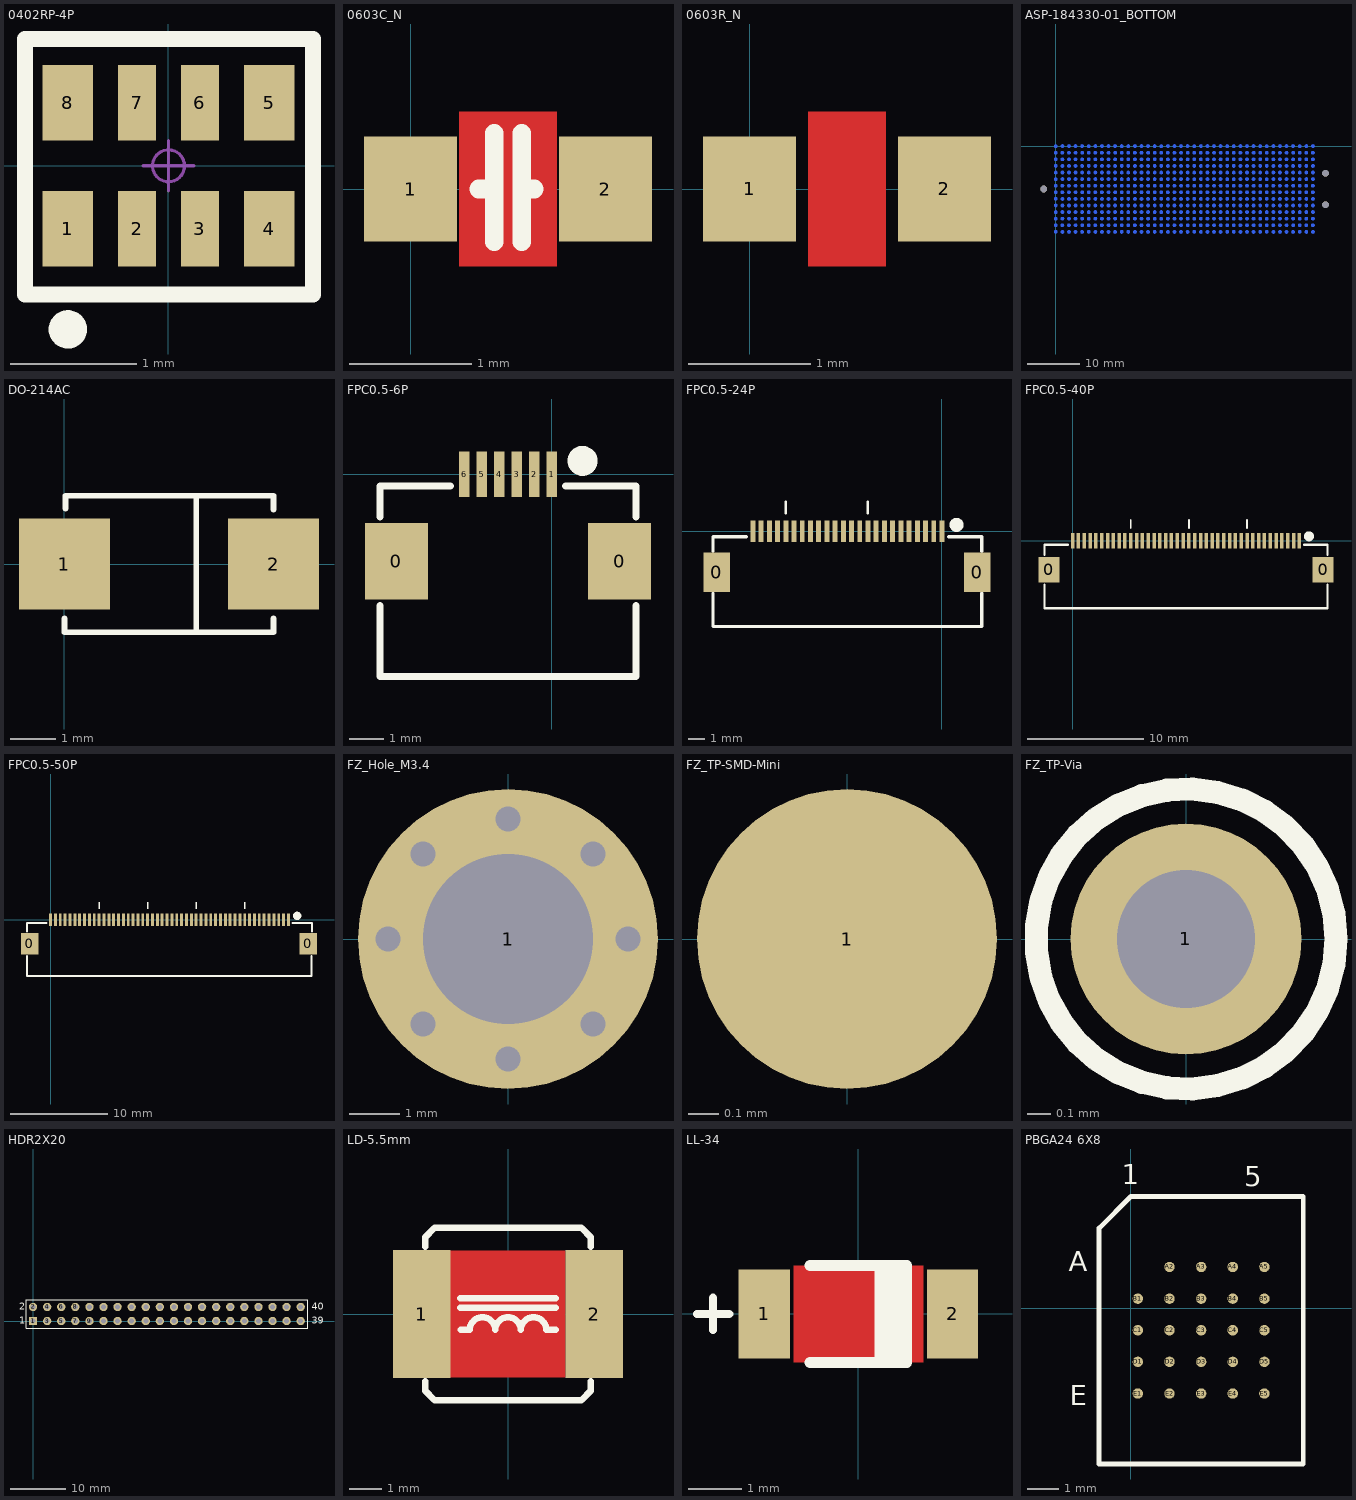
[diagram p0: the footprints below, top view; thin cyan lines are the x and y axes]
# Altium footprint library MISC105414-6.PcbLib: 28 footprints (part 1 of 2)
Each footprint in its own frame and in the unit in brackets; x right, y up, seen from the top. Pads: shape width x height; smd on the part's side, far side on the other; paste and mask are expansions set on the pad; w line width, h text height; cw(c..) or ccw(c..) is an arc to the next point about the centre after c.

## 0402RP-4P [mm] "2mm*1mm*0.45mm(长*宽*厚)"
pads (8):
  rect 0.4x0.6 smd: 1(-0.8,-0.5) 4(0.8,-0.5) 5(0.8,0.5) 8(-0.8,0.5)
  rect 0.3x0.6 smd: 2(-0.25,-0.5) 3(0.25,-0.5) 6(0.25,0.5) 7(-0.25,0.5)
Top Overlay:
  circle w0.152: c-0.8,-1.3 r0.076
  lines w0.127: -1.139,-1.024 -1.139,1.008 1.147,1.008 1.147,-1.024 -1.139,-1.024
Mechanical 15:
  circle w0.025: c0,0 r0.127
  lines w0.025: -0.2,0 0.2,0 ; 0,-0.2 0,0.2
3D body "RCA-8P4R-0402.STEP": height 0.45, standoff 0, extent -1,-0.5 1,0.5

## 0603C_N [mil]
pads (2):
  rect 30x34 smd: 1(-0.01,-0.01) 2(62.99,-0.01)
Top Layer:
  pour cut-out: 15.74,25 47.24,25 47.24,-25 15.74,-25
Top Overlay:
  lines w6: 22,0 27,0 ; 27,-17 27,18 ; 36,-17 36,18 ; 36,0 40,0
3D body "User Library-0603 SMD Capacitor.step": height 12.49, standoff 0.6, extent 0,-15.75 63,15.75

## 0603R_N [mil]
pads (2):
  rect 30x34 smd: 1(0,0) 2(62.99,0)
Top Layer:
  pour cut-out: 19,-25 19,25 44,25 44,-25
3D body "User Library-RESC1608X05N.step": height 17.76, standoff 0, extent 0.01,-16.73 61.03,16.74

## ASP-184330-01_BOTTOM [mm]
pads (560):
  round 0.64 smd far side: A1(0,-2.54) A2(1.27,-2.54) A3(2.54,-2.54) A4(3.81,-2.54) A5(5.08,-2.54) A6(6.35,-2.54) A7(7.62,-2.54) A8(8.89,-2.54) A9(10.16,-2.54) A10(11.43,-2.54) A11(12.7,-2.54) A12(13.97,-2.54) A13(15.24,-2.54) A14(16.51,-2.54) A15(17.78,-2.54) A16(19.05,-2.54) A17(20.32,-2.54) A18(21.59,-2.54) A19(22.86,-2.54) A20(24.13,-2.54) A21(25.4,-2.54) A22(26.67,-2.54) A23(27.94,-2.54) A24(29.21,-2.54) A25(30.48,-2.54) A26(31.75,-2.54) A27(33.02,-2.54) A28(34.29,-2.54) A29(35.56,-2.54) A30(36.83,-2.54) A31(38.1,-2.54) A32(39.37,-2.54) A33(40.64,-2.54) A34(41.91,-2.54) A35(43.18,-2.54) A36(44.45,-2.54) A37(45.72,-2.54) A38(46.99,-2.54) A39(48.26,-2.54) A40(49.53,-2.54) B1(0,-3.81) B2(1.27,-3.81) B3(2.54,-3.81) B4(3.81,-3.81) B5(5.08,-3.81) B6(6.35,-3.81) B7(7.62,-3.81) B8(8.89,-3.81) B9(10.16,-3.81) B10(11.43,-3.81) B11(12.7,-3.81) B12(13.97,-3.81) B13(15.24,-3.81) B14(16.51,-3.81) B15(17.78,-3.81) B16(19.05,-3.81) B17(20.32,-3.81) B18(21.59,-3.81) B19(22.86,-3.81) B20(24.13,-3.81) B21(25.4,-3.81) B22(26.67,-3.81) B23(27.94,-3.81) B24(29.21,-3.81) B25(30.48,-3.81) B26(31.75,-3.81) B27(33.02,-3.81) B28(34.29,-3.81) B29(35.56,-3.81) B30(36.83,-3.81) B31(38.1,-3.81) B32(39.37,-3.81) B33(40.64,-3.81) B34(41.91,-3.81) B35(43.18,-3.81) B36(44.45,-3.81) B37(45.72,-3.81) B38(46.99,-3.81) B39(48.26,-3.81) B40(49.53,-3.81) C1(0,-5.08) C2(1.27,-5.08) C3(2.54,-5.08) C4(3.81,-5.08) C5(5.08,-5.08) C6(6.35,-5.08) C7(7.62,-5.08) C8(8.89,-5.08) C9(10.16,-5.08) C10(11.43,-5.08) C11(12.7,-5.08) C12(13.97,-5.08) C13(15.24,-5.08) C14(16.51,-5.08) C15(17.78,-5.08) C16(19.05,-5.08) C17(20.32,-5.08) C18(21.59,-5.08) C19(22.86,-5.08) C20(24.13,-5.08) C21(25.4,-5.08) C22(26.67,-5.08) C23(27.94,-5.08) C24(29.21,-5.08) C25(30.48,-5.08) C26(31.75,-5.08) C27(33.02,-5.08) C28(34.29,-5.08) C29(35.56,-5.08) C30(36.83,-5.08) C31(38.1,-5.08) C32(39.37,-5.08) C33(40.64,-5.08) C34(41.91,-5.08) C35(43.18,-5.08) C36(44.45,-5.08) C37(45.72,-5.08) C38(46.99,-5.08) C39(48.26,-5.08) C40(49.53,-5.08) D1(0,-6.35) D2(1.27,-6.35) D3(2.54,-6.35) D4(3.81,-6.35) D5(5.08,-6.35) D6(6.35,-6.35) D7(7.62,-6.35) D8(8.89,-6.35) D9(10.16,-6.35) D10(11.43,-6.35) D11(12.7,-6.35) D12(13.97,-6.35) D13(15.24,-6.35) D14(16.51,-6.35) D15(17.78,-6.35) D16(19.05,-6.35) D17(20.32,-6.35) D18(21.59,-6.35) D19(22.86,-6.35) D20(24.13,-6.35) D21(25.4,-6.35) D22(26.67,-6.35) D23(27.94,-6.35) D24(29.21,-6.35) D25(30.48,-6.35) D26(31.75,-6.35) D27(33.02,-6.35) D28(34.29,-6.35) D29(35.56,-6.35) D30(36.83,-6.35) D31(38.1,-6.35) D32(39.37,-6.35) D33(40.64,-6.35) D34(41.91,-6.35) D35(43.18,-6.35) D36(44.45,-6.35) D37(45.72,-6.35) D38(46.99,-6.35) D39(48.26,-6.35) D40(49.53,-6.35) E1(0,-7.62) E2(1.27,-7.62) E3(2.54,-7.62) E4(3.81,-7.62) E5(5.08,-7.62) E6(6.35,-7.62) E7(7.62,-7.62) E8(8.89,-7.62) E9(10.16,-7.62) E10(11.43,-7.62) E11(12.7,-7.62) E12(13.97,-7.62) E13(15.24,-7.62) E14(16.51,-7.62) E15(17.78,-7.62) E16(19.05,-7.62) E17(20.32,-7.62) E18(21.59,-7.62) E19(22.86,-7.62) E20(24.13,-7.62) E21(25.4,-7.62) E22(26.67,-7.62) E23(27.94,-7.62) E24(29.21,-7.62) E25(30.48,-7.62) E26(31.75,-7.62) E27(33.02,-7.62) E28(34.29,-7.62) E29(35.56,-7.62) E30(36.83,-7.62) E31(38.1,-7.62) E32(39.37,-7.62) E33(40.64,-7.62) E34(41.91,-7.62) E35(43.18,-7.62) E36(44.45,-7.62) E37(45.72,-7.62) E38(46.99,-7.62) E39(48.26,-7.62) E40(49.53,-7.62) F1(0,-8.89) F2(1.27,-8.89) F3(2.54,-8.89) F4(3.81,-8.89) F5(5.08,-8.89) F6(6.35,-8.89) F7(7.62,-8.89) F8(8.89,-8.89) F9(10.16,-8.89) F10(11.43,-8.89) F11(12.7,-8.89) F12(13.97,-8.89) F13(15.24,-8.89) F14(16.51,-8.89) F15(17.78,-8.89) F16(19.05,-8.89) F17(20.32,-8.89) F18(21.59,-8.89) F19(22.86,-8.89) F20(24.13,-8.89) F21(25.4,-8.89) F22(26.67,-8.89) F23(27.94,-8.89) F24(29.21,-8.89) F25(30.48,-8.89) F26(31.75,-8.89) F27(33.02,-8.89) F28(34.29,-8.89) F29(35.56,-8.89) F30(36.83,-8.89) F31(38.1,-8.89) F32(39.37,-8.89) F33(40.64,-8.89) F34(41.91,-8.89) F35(43.18,-8.89) F36(44.45,-8.89) F37(45.72,-8.89) F38(46.99,-8.89) F39(48.26,-8.89) F40(49.53,-8.89) G1(0,-10.16) G2(1.27,-10.16) G3(2.54,-10.16) G4(3.81,-10.16) G5(5.08,-10.16) G6(6.35,-10.16) G7(7.62,-10.16) G8(8.89,-10.16) G9(10.16,-10.16) G10(11.43,-10.16) G11(12.7,-10.16) G12(13.97,-10.16) G13(15.24,-10.16) G14(16.51,-10.16) G15(17.78,-10.16) G16(19.05,-10.16) G17(20.32,-10.16) G18(21.59,-10.16) G19(22.86,-10.16) G20(24.13,-10.16) G21(25.4,-10.16) G22(26.67,-10.16) G23(27.94,-10.16) G24(29.21,-10.16) G25(30.48,-10.16) G26(31.75,-10.16) G27(33.02,-10.16) G28(34.29,-10.16) G29(35.56,-10.16) G30(36.83,-10.16) G31(38.1,-10.16) G32(39.37,-10.16) G33(40.64,-10.16) G34(41.91,-10.16) G35(43.18,-10.16) G36(44.45,-10.16) G37(45.72,-10.16) G38(46.99,-10.16) G39(48.26,-10.16) G40(49.53,-10.16) H1(0,-11.43) H2(1.27,-11.43) H3(2.54,-11.43) H4(3.81,-11.43) H5(5.08,-11.43) H6(6.35,-11.43) H7(7.62,-11.43) H8(8.89,-11.43) H9(10.16,-11.43) H10(11.43,-11.43) H11(12.7,-11.43) H12(13.97,-11.43) H13(15.24,-11.43) H14(16.51,-11.43) H15(17.78,-11.43) H16(19.05,-11.43) H17(20.32,-11.43) H18(21.59,-11.43) H19(22.86,-11.43) H20(24.13,-11.43) H21(25.4,-11.43) H22(26.67,-11.43) H23(27.94,-11.43) H24(29.21,-11.43) H25(30.48,-11.43) H26(31.75,-11.43) H27(33.02,-11.43) H28(34.29,-11.43) H29(35.56,-11.43) H30(36.83,-11.43) H31(38.1,-11.43) H32(39.37,-11.43) H33(40.64,-11.43) H34(41.91,-11.43) H35(43.18,-11.43) H36(44.45,-11.43) H37(45.72,-11.43) H38(46.99,-11.43) H39(48.26,-11.43) H40(49.53,-11.43) J1(0,-12.7) J2(1.27,-12.7) J3(2.54,-12.7) J4(3.81,-12.7) J5(5.08,-12.7) J6(6.35,-12.7) J7(7.62,-12.7) J8(8.89,-12.7) J9(10.16,-12.7) J10(11.43,-12.7) J11(12.7,-12.7) J12(13.97,-12.7) J13(15.24,-12.7) J14(16.51,-12.7) J15(17.78,-12.7) J16(19.05,-12.7) J17(20.32,-12.7) J18(21.59,-12.7) J19(22.86,-12.7) J20(24.13,-12.7) J21(25.4,-12.7) J22(26.67,-12.7) J23(27.94,-12.7) J24(29.21,-12.7) J25(30.48,-12.7) J26(31.75,-12.7) J27(33.02,-12.7) J28(34.29,-12.7) J29(35.56,-12.7) J30(36.83,-12.7) J31(38.1,-12.7) J32(39.37,-12.7) J33(40.64,-12.7) J34(41.91,-12.7) J35(43.18,-12.7) J36(44.45,-12.7) J37(45.72,-12.7) J38(46.99,-12.7) J39(48.26,-12.7) J40(49.53,-12.7) K1(0,-13.97) K2(1.27,-13.97) K3(2.54,-13.97) K4(3.81,-13.97) K5(5.08,-13.97) K6(6.35,-13.97) K7(7.62,-13.97) K8(8.89,-13.97) K9(10.16,-13.97) K10(11.43,-13.97) K11(12.7,-13.97) K12(13.97,-13.97) K13(15.24,-13.97) K14(16.51,-13.97) K15(17.78,-13.97) K16(19.05,-13.97) K17(20.32,-13.97) K18(21.59,-13.97) K19(22.86,-13.97) K20(24.13,-13.97) K21(25.4,-13.97) K22(26.67,-13.97) K23(27.94,-13.97) K24(29.21,-13.97) K25(30.48,-13.97) K26(31.75,-13.97) K27(33.02,-13.97) K28(34.29,-13.97) K29(35.56,-13.97) K30(36.83,-13.97) K31(38.1,-13.97) K32(39.37,-13.97) K33(40.64,-13.97) K34(41.91,-13.97) K35(43.18,-13.97) K36(44.45,-13.97) K37(45.72,-13.97) K38(46.99,-13.97) K39(48.26,-13.97) K40(49.53,-13.97) L1(0,-15.24) L2(1.27,-15.24) L3(2.54,-15.24) L4(3.81,-15.24) L5(5.08,-15.24) L6(6.35,-15.24) L7(7.62,-15.24) L8(8.89,-15.24) L9(10.16,-15.24) L10(11.43,-15.24) L11(12.7,-15.24) L12(13.97,-15.24) L13(15.24,-15.24) L14(16.51,-15.24) L15(17.78,-15.24) L16(19.05,-15.24) L17(20.32,-15.24) L18(21.59,-15.24) L19(22.86,-15.24) L20(24.13,-15.24) L21(25.4,-15.24) L22(26.67,-15.24) L23(27.94,-15.24) L24(29.21,-15.24) L25(30.48,-15.24) L26(31.75,-15.24) L27(33.02,-15.24) L28(34.29,-15.24) L29(35.56,-15.24) L30(36.83,-15.24) L31(38.1,-15.24) L32(39.37,-15.24) L33(40.64,-15.24) L34(41.91,-15.24) L35(43.18,-15.24) L36(44.45,-15.24) L37(45.72,-15.24) L38(46.99,-15.24) L39(48.26,-15.24) L40(49.53,-15.24) M1(0,-16.51) M2(1.27,-16.51) M3(2.54,-16.51) M4(3.81,-16.51) M5(5.08,-16.51) M6(6.35,-16.51) M7(7.62,-16.51) M8(8.89,-16.51) M9(10.16,-16.51) M10(11.43,-16.51) M11(12.7,-16.51) M12(13.97,-16.51) M13(15.24,-16.51) M14(16.51,-16.51) M15(17.78,-16.51) M16(19.05,-16.51) M17(20.32,-16.51) M18(21.59,-16.51) M19(22.86,-16.51) M20(24.13,-16.51) M21(25.4,-16.51) M22(26.67,-16.51) M23(27.94,-16.51) M24(29.21,-16.51) M25(30.48,-16.51) M26(31.75,-16.51) M27(33.02,-16.51) M28(34.29,-16.51) M29(35.56,-16.51) M30(36.83,-16.51) M31(38.1,-16.51) M32(39.37,-16.51) M33(40.64,-16.51) M34(41.91,-16.51) M35(43.18,-16.51) M36(44.45,-16.51) M37(45.72,-16.51) M38(46.99,-16.51) M39(48.26,-16.51) M40(49.53,-16.51) Y1(0,0) Y2(1.27,0) Y3(2.54,0) Y4(3.81,0) Y5(5.08,0) Y6(6.35,0) Y7(7.62,0) Y8(8.89,0) Y9(10.16,0) Y10(11.43,0) Y11(12.7,0) Y12(13.97,0) Y13(15.24,0) Y14(16.51,0) Y15(17.78,0) Y16(19.05,0) Y17(20.32,0) Y18(21.59,0) Y19(22.86,0) Y20(24.13,0) Y21(25.4,0) Y22(26.67,0) Y23(27.94,0) Y24(29.21,0) Y25(30.48,0) Y26(31.75,0) Y27(33.02,0) Y28(34.29,0) Y29(35.56,0) Y30(36.83,0) Y31(38.1,0) Y32(39.37,0) Y33(40.64,0) Y34(41.91,0) Y35(43.18,0) Y36(44.45,0) Y37(45.72,0) Y38(46.99,0) Y39(48.26,0) Y40(49.53,0) Z1(0,-1.27) Z2(1.27,-1.27) Z3(2.54,-1.27) Z4(3.81,-1.27) Z5(5.08,-1.27) Z6(6.35,-1.27) Z7(7.62,-1.27) Z8(8.89,-1.27) Z9(10.16,-1.27) Z10(11.43,-1.27) Z11(12.7,-1.27) Z12(13.97,-1.27) Z13(15.24,-1.27) Z14(16.51,-1.27) Z15(17.78,-1.27) Z16(19.05,-1.27) Z17(20.32,-1.27) Z18(21.59,-1.27) Z19(22.86,-1.27) Z20(24.13,-1.27) Z21(25.4,-1.27) Z22(26.67,-1.27) Z23(27.94,-1.27) Z24(29.21,-1.27) Z25(30.48,-1.27) Z26(31.75,-1.27) Z27(33.02,-1.27) Z28(34.29,-1.27) Z29(35.56,-1.27) Z30(36.83,-1.27) Z31(38.1,-1.27) Z32(39.37,-1.27) Z33(40.64,-1.27) Z34(41.91,-1.27) Z35(43.18,-1.27) Z36(44.45,-1.27) Z37(45.72,-1.27) Z38(46.99,-1.27) Z39(48.26,-1.27) Z40(49.53,-1.27)
via -2.311,-8.255 diameter 1.3 hole 1.3
via 51.968,-5.207 diameter 1.3 hole 1.3
via 51.968,-11.303 diameter 1.3 hole 1.3
Bottom Overlay:
  lines w0.2: -3.81,-11.811 -3.048,-11.811 -3.048,-17.78 53.975,-17.78 53.975,1.27 -3.048,1.27 -3.048,-4.699 -3.81,-4.699 -3.81,-11.811

## DO-214AC [mm]
pads (2):
  rect 2x2 smd: 1(0,0) 2(4.6,0)
Top Overlay:
  lines w0.127: 0,-1.2 0,-1.5 4.6,-1.5 4.6,-1.2 ; 0.02,1.22 0.02,1.5 4.6,1.5 4.6,1.2 ; 2.9,-1.5 2.9,1.5

## FPC0.5-6P [mm]
pads (8):
  rect 1.8x2.2 smd: 0(-4.45,-2.497) 0(1.95,-2.497)
  rect 0.3x1.3 smd: 1(0,0) 2(-0.5,0) 3(-1,0) 4(-1.5,0) 5(-2,0) 6(-2.5,0)
Top Overlay:
  circle w0.5: c0.889,0.381 r0.18
  lines w0.2: -4.925,-3.767 -4.925,-5.799 2.425,-5.799 2.425,-3.767 ; -4.925,-1.227 -4.925,-0.338 -2.893,-0.338 ; 0.393,-0.338 2.425,-0.338 2.425,-1.227
3D body "FPC0.5-6P.STEP": height 2, standoff -0.01, extent -4.85,-5.545 2.35,0.455

## FPC0.5-24P [mm]
pads (26):
  rect 1.6x2.4 smd: 0(-13.704,-2.497) 0(2.15,-2.497)
  rect 0.3x1.3 smd: 1(0,0) 2(-0.5,0) 3(-1,0) 4(-1.5,0) 5(-2,0) 6(-2.5,0) 7(-3,0) 8(-3.5,0) 9(-4,0) 10(-4.5,0) 11(-5,0) 12(-5.5,0) 13(-6,0) 14(-6.5,0) 15(-7,0) 16(-7.5,0) 17(-8,0) 18(-8.5,0) 19(-9,0) 20(-9.5,0) 21(-10,0) 22(-10.5,0) 23(-11,0) 24(-11.5,0)
Top Overlay:
  circle w0.5: c0.889,0.381 r0.18
  lines w0.152: -9.5,1.1 -9.5,1.8 ; -4.5,1.1 -4.5,1.8
  lines w0.2: -13.925,-3.767 -13.925,-5.799 2.425,-5.799 2.425,-3.767 ; -13.925,-1.227 -13.925,-0.338 -11.893,-0.338 ; 0.393,-0.338 2.425,-0.338 2.425,-1.227
3D body "FPC0.5-24P.STEP": height 2, standoff -0.01, extent -13.853,-5.7 2.347,0.3

## FPC0.5-40P [mm]
pads (42):
  rect 1.8x2.2 smd: 0(-2.05,-2.497) 0(21.55,-2.497)
  rect 0.3x1.3 smd: 1(19.5,0) 2(19,0) 3(18.5,0) 4(18,0) 5(17.5,0) 6(17,0) 7(16.5,0) 8(16,0) 9(15.5,0) 10(15,0) 11(14.5,0) 12(14,0) 13(13.5,0) 14(13,0) 15(12.5,0) 16(12,0) 17(11.5,0) 18(11,0) 19(10.5,0) 20(10,0) 21(9.5,0) 22(9,0) 23(8.5,0) 24(8,0) 25(7.5,0) 26(7,0) 27(6.5,0) 28(6,0) 29(5.5,0) 30(5,0) 31(4.5,0) 32(4,0) 33(3.5,0) 34(3,0) 35(2.5,0) 36(2,0) 37(1.5,0) 38(1,0) 39(0.5,0) 40(0,0)
Top Overlay:
  circle w0.5: c20.32,0.381 r0.18
  lines w0.152: 5,1.1 5,1.8 ; 10,1.1 10,1.8 ; 15,1.1 15,1.8
  lines w0.2: -2.425,-3.767 -2.425,-5.799 21.925,-5.799 21.925,-3.767 ; -2.425,-1.227 -2.425,-0.338 -0.393,-0.338 ; 19.893,-0.338 21.925,-0.338 21.925,-1.227
3D body "FPC0.5-40P.STEP": height 2, standoff -0.01, extent -2.34,-5.726 21.86,0.274

## FPC0.5-50P [mm] "FPCTOP;0.5mm;"
height 1
pads (52):
  rect 1.8x2.2 smd: 0(-2.15,-2.497) 0(26.55,-2.497)
  rect 0.3x1.3 smd: 1(24.5,0) 2(24,0) 3(23.5,0) 4(23,0) 5(22.5,0) 6(22,0) 7(21.5,0) 8(21,0) 9(20.5,0) 10(20,0) 11(19.5,0) 12(19,0) 13(18.5,0) 14(18,0) 15(17.5,0) 16(17,0) 17(16.5,0) 18(16,0) 19(15.5,0) 20(15,0) 21(14.5,0) 22(14,0) 23(13.5,0) 24(13,0) 25(12.5,0) 26(12,0) 27(11.5,0) 28(11,0) 29(10.5,0) 30(10,0) 31(9.5,0) 32(9,0) 33(8.5,0) 34(8,0) 35(7.5,0) 36(7,0) 37(6.5,0) 38(6,0) 39(5.5,0) 40(5,0) 41(4.5,0) 42(4,0) 43(3.5,0) 44(3,0) 45(2.5,0) 46(2,0) 47(1.5,0) 48(1,0) 49(0.5,0) 50(0,0)
Top Overlay:
  circle w0.5: c25.4,0.381 r0.18
  lines w0.152: 5,1.1 5,1.8 ; 10,1.1 10,1.8 ; 15,1.1 15,1.8 ; 20,1.1 20,1.8
  lines w0.2: -2.425,-3.767 -2.425,-5.799 26.9,-5.799 26.9,-3.767 ; -2.425,-1.227 -2.425,-0.338 -0.393,-0.338 ; 24.893,-0.338 26.925,-0.338 26.925,-1.227

## FZ_Hole_M3.4 [mm]
pads (1):
  round 6 hole 3.4: 1(0,0)
via 0,2.4 diameter 1 hole 0.5
via 0,2.4 diameter 1 hole 0.5
via -1.697,1.697 diameter 1 hole 0.5
via -2.4,0 diameter 1 hole 0.5
via -1.697,-1.697 diameter 1 hole 0.5
via 0,-2.4 diameter 1 hole 0.5
via 1.697,-1.697 diameter 1 hole 0.5
via 2.4,0 diameter 1 hole 0.5
via 1.697,1.697 diameter 1 hole 0.5

## FZ_TP-SMD-Mini [mm]
pads (1):
  round 1 smd mask+0.05: 1(0,0)

## FZ_TP-Via [mm]
pads (1):
  round 1 hole 0.6 mask+0.1: 1(0,0)
Top Overlay:
  circle w0.1: c0,0 r0.65

## HDR2X20 [mm] "Connector; Header; 20x2 Position"
pads (40):
  rect 1.5x1.5 hole 0.9: 1(0,0)
  round 1.5 hole 0.9: 2(0,2.54) 3(2.54,0) 4(2.54,2.54) 5(5.08,0) 6(5.08,2.54) 7(7.62,0) 8(7.62,2.54) 9(10.16,0) 10(10.16,2.54) 11(12.7,0) 12(12.7,2.54) 13(15.24,0) 14(15.24,2.54) 15(17.78,0) 16(17.78,2.54) 17(20.32,0) 18(20.32,2.54) 19(22.86,0) 20(22.86,2.54) 21(25.4,0) 22(25.4,2.54) 23(27.94,0) 24(27.94,2.54) 25(30.48,0) 26(30.48,2.54) 27(33.02,0) 28(33.02,2.54) 29(35.56,0) 30(35.56,2.54) 31(38.1,0) 32(38.1,2.54) 33(40.64,0) 34(40.64,2.54) 35(43.18,0) 36(43.18,2.54) 37(45.72,0) 38(45.72,2.54) 39(48.26,0) 40(48.26,2.54)
Top Overlay:
  lines w0.2: -1.27,-1.27 49.53,-1.27 49.53,3.81 -1.27,3.81 -1.27,-1.27
  text "1" at -2.54,-0.508 h1.27
  text "2" at -2.54,2.032 h1.27
  text "40" at 50.292,2.032 h1.27
  text "39" at 50.292,-0.508 h1.27

## LD-5.5mm [mm]
pads (2):
  rect 1.8x4 smd: 1(-2.7,0) 2(2.7,0)
Top Layer:
  pour cut-out: -1.841,-1.978 -1.841,1.978 1.8,1.978 1.8,-1.978
Top Overlay:
  lines w0.203: -2.6,-2.1 -2.6,-2.4 -2.3,-2.7 2.3,-2.7 2.6,-2.4 2.6,-2.1 ; -2.6,2.1 -2.6,2.4 -2.3,2.7 2.3,2.7 2.6,2.4 2.6,2.1 ; -1.5,0.2 1.5,0.2 ; -1.5,0.5 1.5,0.5 ; -1.477,-0.5 -1.2,-0.5 cw(c-0.8,-0.5) -0.4,-0.5 cw(c0,-0.5) 0.4,-0.5 cw(c0.8,-0.5) 1.2,-0.5 1.5,-0.5

## LL-34 [mm]
pads (2):
  rect 0.95x1.65 smd: 1(-1.75,0) 2(1.75,0)
Top Layer:
  pour cut-out: -1.2,0.9 1.2,0.9 1.2,-0.9 -1.2,-0.9
Top Overlay:
  rectangle: 0.3,-0.9 0.9,0.9
  lines w0.152: -3,0 -2.4,0 ; -2.7,-0.3 -2.7,0.3
  lines w0.2: -0.9,-0.9 0.9,-0.9 0.9,0.9 -0.9,0.9

## PBGA24 6X8 [mil]
pads (24):
  round 13 smd: A2(47.95,51.06) A3(87.32,51.06) A4(126.69,51.06) A5(166.06,51.06) B1(8.58,11.69) B2(47.95,11.69) B3(87.32,11.69) B4(126.69,11.69) B5(166.06,11.69) C1(8.58,-27.68) C2(47.95,-27.68) C3(87.32,-27.68) C4(126.69,-27.68) C5(166.06,-27.68) D1(8.58,-67.05) D2(47.95,-67.05) D3(87.32,-67.05) D4(126.69,-67.05) D5(166.06,-67.05) E1(8.58,-106.42) E2(47.95,-106.42) E3(87.32,-106.42) E4(126.69,-106.42) E5(166.06,-106.42)
Top Overlay:
  lines w6: -39.76,-194.13 -39.76,99.4 -0.39,138.77 214.4,138.77 214.4,-194.13 -39.76,-194.13
  text "A" at -77.46,45.8 h25
  text "E" at -76.1,-121.06 h25
  text "1" at -11.59,154.21 h25
  text "5" at 140.82,151.32 h25
Mechanical 15:
  text "C5" at 144.79,-32.71 h15
  text "B5" at 144.79,6.66 h15
  text "A5" at 144.79,46.03 h15
  text "A2" at 26.68,46.03 h15
  text "A3" at 66.05,46.03 h15
  text "C3" at 66.05,-32.71 h15
  text "C4" at 105.42,-32.71 h15
  text "D4" at 105.42,-72.08 h15
  text "D2" at 26.68,-72.08 h15
  text "D3" at 66.05,-72.08 h15
  text "B2" at 26.68,6.66 h15
  text "C2" at 26.68,-32.71 h15
  text "D5" at 144.79,-72.08 h15
  text "E3" at 66.05,-111.45 h15
  text "E2" at 26.68,-111.45 h15
  text "E1" at -12.69,-111.45 h15
  text "B1" at -12.69,6.66 h15
  text "E4" at 105.42,-111.45 h15
  text "D1" at -12.69,-72.08 h15
  text "B4" at 105.42,6.66 h15
  text "A4" at 105.42,46.03 h15
  text "C1" at -12.69,-32.71 h15
  text "E5" at 144.79,-111.45 h15
  text "B3" at 66.05,6.66 h15